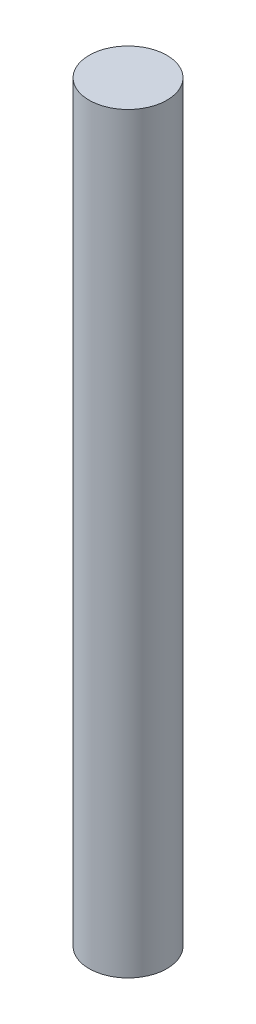
SolidWorks part; units mm, degrees
ref_plane "前视基准面" through (0, 0, 0) normal (0, 0, 1) x (1, 0, 0)
ref_plane "上视基准面" through (0, 0, 0) normal (0, 1, 0) x (1, 0, 0)
ref_plane "右视基准面" through (0, 0, 0) normal (1, 0, 0) x (0, 0, -1)
sketch "草图1" plane through (0, 0, 0) normal (0, 1, 0) x (1, 0, 0)
  circle A0 centre (0, 0) radius 3
  circle A1 centre (0, 0) radius 1.5
extrude "凸台-拉伸1" add sketch "草图1" along normal blind 58 contours A0 A1 | A1
